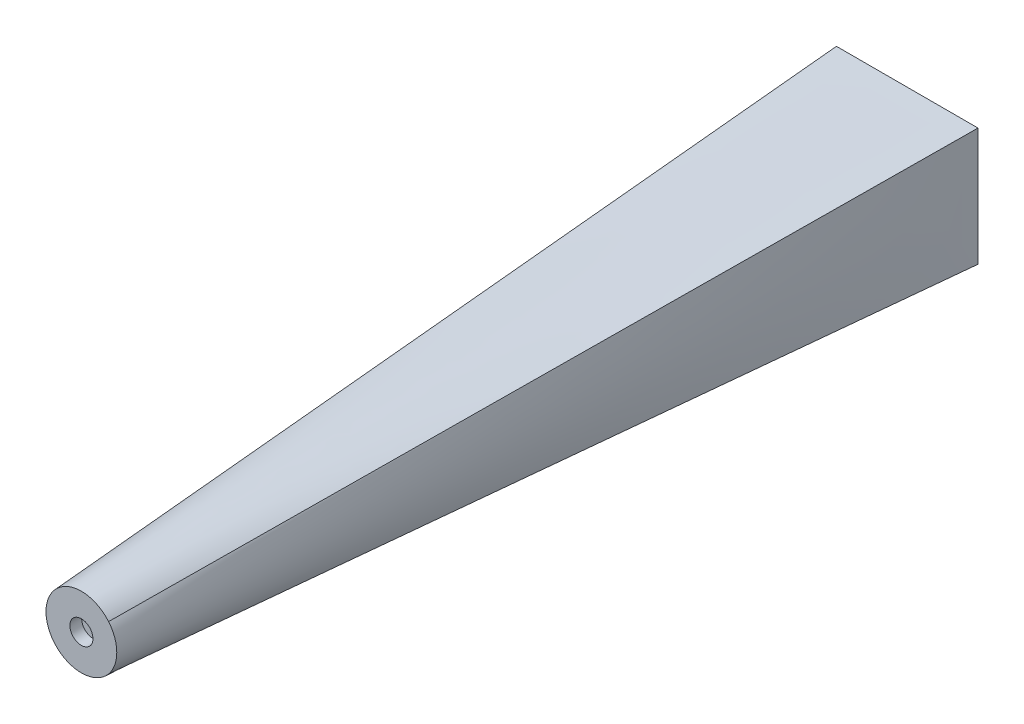
from build123d import *

# Parameters (mm, degrees)
SKETCH_3_R          = 4.889549894
CUT_EXTRUDE_1_DEPTH = 5


with BuildPart() as part:
    # 草图2 → 放样1 section 0
    with BuildSketch(Plane.XY.offset(-350)):
        with BuildLine():
            Line((-30, 25), (30, 25))
            Line((30, 25), (30, -25))
            Line((30, -25), (-30, -25))
            Line((-30, -25), (-30, 25))
        make_face()
    # 草图1 for 放样1 → 放样1 section 1
    with BuildSketch(Plane.XY):
        with BuildLine():
            # circular arc as an exact rational Bezier (weights 1, cos(half-angle), 1)
            Bezier((-11.523319194, 9.602765995), (0, 23.430749028), (11.523319194, 9.602765995), weights=[1, 0.6401844, 1])
            Bezier((11.523319194, 9.602765995), (19.52562419, 0), (11.523319194, -9.602765995), weights=[1, 0.76822128, 1])
            Bezier((11.523319194, -9.602765995), (0, -23.430749028), (-11.523319194, -9.602765995), weights=[1, 0.6401844, 1])
            Bezier((-11.523319194, -9.602765995), (-19.52562419, 0), (-11.523319194, 9.602765995), weights=[1, 0.76822128, 1])
        make_face()
    loft()

    # 草图3 → 切除-拉伸1 (cut)
    with BuildSketch(Plane.XY):
        Circle(SKETCH_3_R)
    extrude(amount=-CUT_EXTRUDE_1_DEPTH, mode=Mode.SUBTRACT)


solid = part.part
